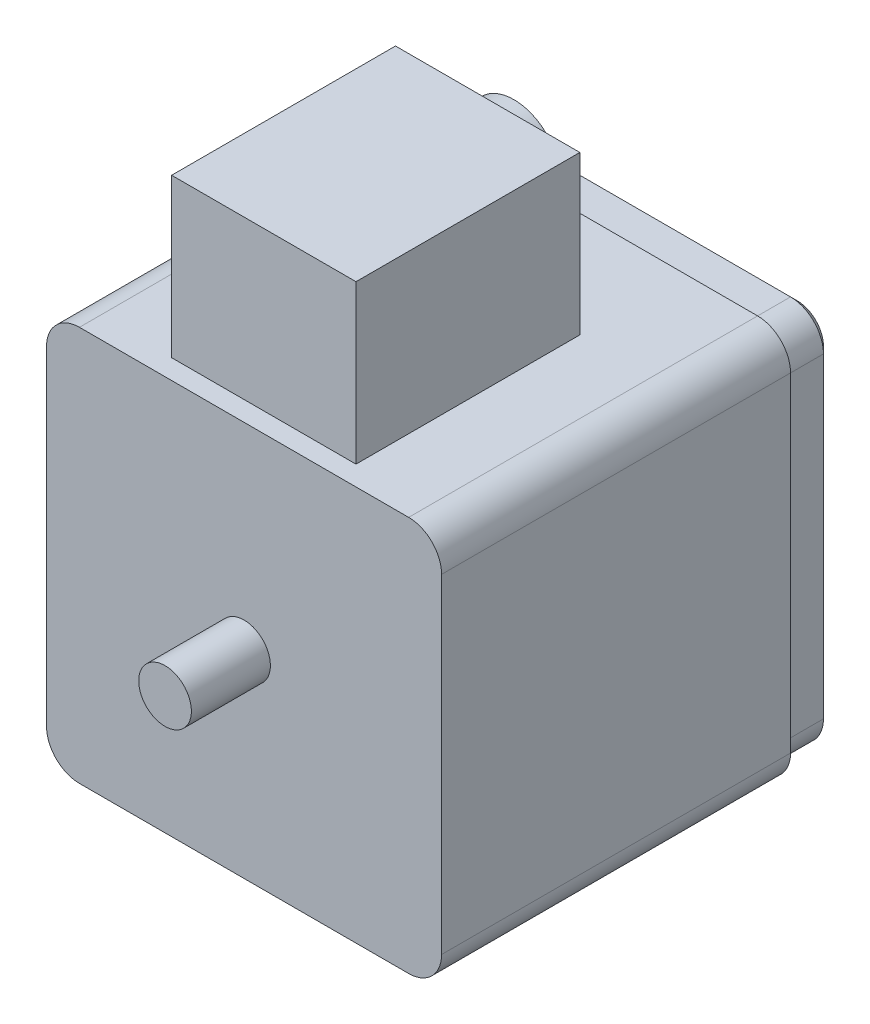
SolidWorks part; units mm, degrees
ref_plane "前视基准面" through (0, 0, 0) normal (0, 0, 1) x (1, 0, 0)
ref_plane "上视基准面" through (0, 0, 0) normal (0, 1, 0) x (1, 0, 0)
ref_plane "右视基准面" through (0, 0, 0) normal (1, 0, 0) x (0, 0, -1)
other "Configuration Table"
sketch "草图1" plane through (0, 0, 0) normal (0, 0, 1) x (1, 0, 0)
  line L1 (-30, 30) -> (30, 30)
  line L2 (-30, 30) -> (-30, -30)
  line L3 (-30, -30) -> (30, -30)
  line L4 (30, 30) -> (30, -30)
  line L5 (-30, 30) -> (30, -30) construction
  line L6 (-30, -30) -> (30, 30) construction
  point P0 (0, 0)
extrude "凸台-拉伸1" add sketch "草图1" along normal blind 60
sketch "草图3" plane through (0, 0, 60) normal (0, 0, 1) x (1, 0, 0)
  circle A0 centre (0, 0) radius 4
extrude "凸台-拉伸2" add sketch "草图3" along normal blind 12
sketch "草图4" plane through (0, 0, 0) normal (0, 0, -1) x (-1, 0, 0)
  line L1 (-29, 29) -> (29, 29)
  line L2 (-29, 29) -> (-29, -29)
  line L3 (-29, -29) -> (29, -29)
  line L4 (29, 29) -> (29, -29)
  line L5 (-29, 29) -> (29, -29) construction
  line L6 (-29, -29) -> (29, 29) construction
  line L8 (-30, 30) -> (30, 30)
  line L9 (-30, 30) -> (-30, -30)
  line L10 (-30, -30) -> (30, -30)
  line L11 (30, 30) -> (30, -30)
  line L12 (-30, 30) -> (30, -30) construction
  line L13 (-30, -30) -> (30, 30) construction
  point P1 (0, 0)
  point P8 (0, 0)
extrude "切除-拉伸4" cut sketch "草图4" against normal blind 7
fillet "圆角4" radius 5 4 edges at (29, 29, 3.5) (-29, 29, 3.5) (-29, -29, 3.5) (29, -29, 3.5)
chamfer "倒角1" distance 1 angle 45 8 edges at (-27.5355, -27.5355, 0) (-29, 0, 0) (0, -29, 0) (-27.5355, 27.5355, 0) (27.5355, -27.5355, 0) (0, 29, 0) (29, 0, 0) (27.5355, 27.5355, 0)
sketch "草图6" plane through (0, 0, 60) normal (0, 0, 1) x (1, 0, 0)
  line L1 (-30, 30) -> (30, 30)
  line L2 (-30, 30) -> (-30, -30)
  line L3 (-30, -30) -> (30, -30)
  line L4 (30, 30) -> (30, -30)
  line L5 (-30, 30) -> (30, -30) construction
  line L6 (-30, -30) -> (30, 30) construction
  point P0 (0, 0)
fillet "圆角6" radius 5 4 edges at (30, -30, 33.5) (-30, -30, 33.5) (-30, 30, 33.5) (30, 30, 33.5)
ref_plane "基准面2" through (0, 30, 0) normal (0, 1, 0) x (1, 0, 0)
sketch "草图7" plane through (0, 30, 0) normal (0, 1, 0) x (1, 0, 0)
  line L0 (0, 5.5563) -> (0, -74.3658) construction
  line L1 (-32.1493, -57) -> (39.9565, -57) construction
  line L2 (-30, -60) -> (30, -60) construction
  line L3 (14, -57) -> (-14, -57)
  line L4 (-14, -57) -> (-14, -19)
  line L5 (-14, -19) -> (14, -19)
  line L6 (14, -57) -> (14, -19)
  point P12 (0, -57)
  point P13 (0, -19)
  dimension "D1" = 3
extrude "凸台-拉伸3" add sketch "草图7" along normal blind 24
sketch "草图8" plane through (0, 0, 19) normal (0, 0, -1) x (-1, 0, 0)
  line L0 (0, 56.3608) -> (0, -9.3145) construction
  line L1 (30, 30) -> (-30, 30) construction
  line L2 (-22.114, 59.89) -> (22.114, 59.89)
  line L3 (-22.114, 59.89) -> (-22.114, 30)
  line L4 (-22.114, 30) -> (22.114, 30)
  line L5 (22.114, 59.89) -> (22.114, 30)
  line L6 (-22.114, 59.89) -> (22.114, 30) construction
  line L7 (-22.114, 30) -> (22.114, 59.89) construction
  circle A0 centre (0, 44.945) radius 7
  point P3 (0, 44.945)
extrude "切除-拉伸5" cut sketch "草图8" against normal blind 4
